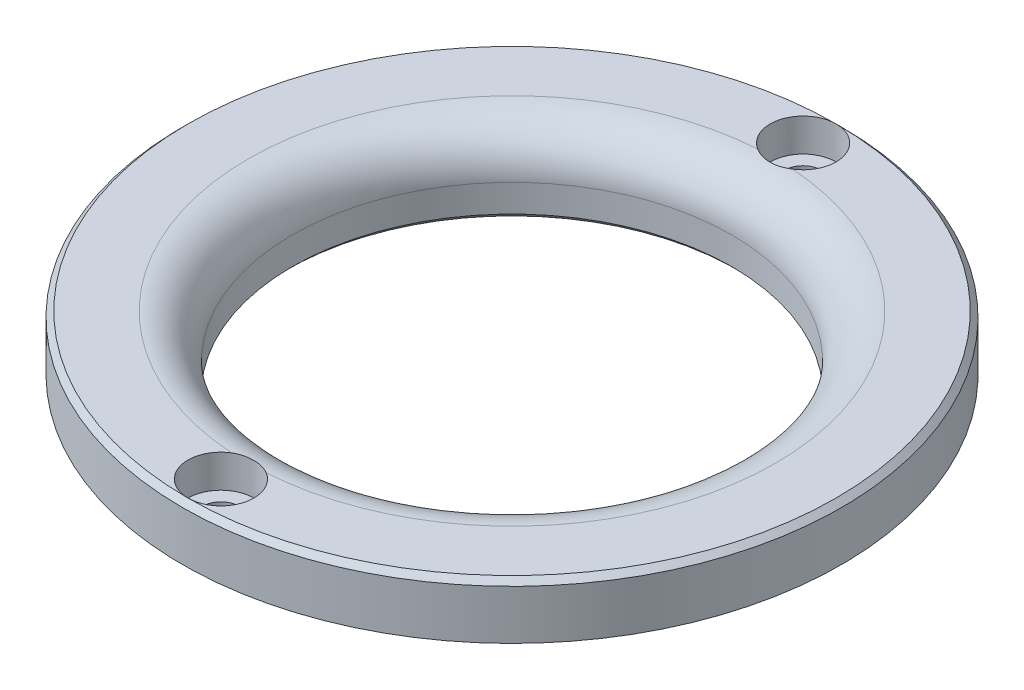
from build123d import *

# Parameters (mm, degrees)
SKETCH_1_R                = 30
SKETCH_1_R_2              = 20
EXTRUDE_1_DEPTH           = 3.5
SKETCH_2_OUTSIDE_W        = 79.028
SKETCH_2_OUTSIDE_H        = 79.028
SKETCH_2_OUTSIDE_R        = 23
CUT_EXTRUDE_1_DEPTH       = 2
FILLET_1_R                = 4
CHAMFER_1_SIZE            = 0.5
HOLE_WIZARD_1_D           = 3.4
HOLE_WIZARD_1_CBORE_D     = 6
HOLE_WIZARD_1_CBORE_DEPTH = 3


with BuildPart() as part:
    # 草图1 → 凸台-拉伸1 (new, symmetric)
    with BuildSketch(Plane(origin=(0, 0, 0), x_dir=(1, 0, 0), z_dir=(0, 1, 0))):
        with Locations(Location((0, 0, 0), (0, 0, 270))):
            Circle(SKETCH_1_R)
        with Locations(Location((0, 0, 0), (0, 0, 270))):
            Circle(SKETCH_1_R_2, mode=Mode.SUBTRACT)
    extrude(amount=EXTRUDE_1_DEPTH, both=True)

    # 草图2 outside → 切除-拉伸1 (cut)
    with BuildSketch(Plane.XZ.offset(3.5)):
        Rectangle(SKETCH_2_OUTSIDE_W, SKETCH_2_OUTSIDE_H)
        with Locations(Location((0, 0, 0), (0, 0, 270))):
            Circle(SKETCH_2_OUTSIDE_R, mode=Mode.SUBTRACT)
    extrude(amount=-CUT_EXTRUDE_1_DEPTH, mode=Mode.SUBTRACT)

    # 圆角1
    fillet_1_edges = [part.edges().sort_by_distance(p)[0] for p in [
        (0, 3.5, -20),
    ]]
    fillet(fillet_1_edges, radius=FILLET_1_R)

    # 倒角1
    chamfer_1_edges = [part.edges().sort_by_distance(p)[0] for p in [
        (0, -3.5, 23),
        (0, 3.5, -30),
        (0, -3.5, -20),
    ]]
    chamfer(chamfer_1_edges, length=CHAMFER_1_SIZE)

    # 打孔尺寸根据内六角圆柱头螺钉的类型1 (through all)
    with Locations(Plane(origin=(0, 3.5, 0), x_dir=(1, 0, 0), z_dir=(0, 1, 0))):
        with Locations((0, -26.5), (0, 26.5)):
            CounterBoreHole(HOLE_WIZARD_1_D / 2, HOLE_WIZARD_1_CBORE_D / 2, HOLE_WIZARD_1_CBORE_DEPTH)


solid = part.part
